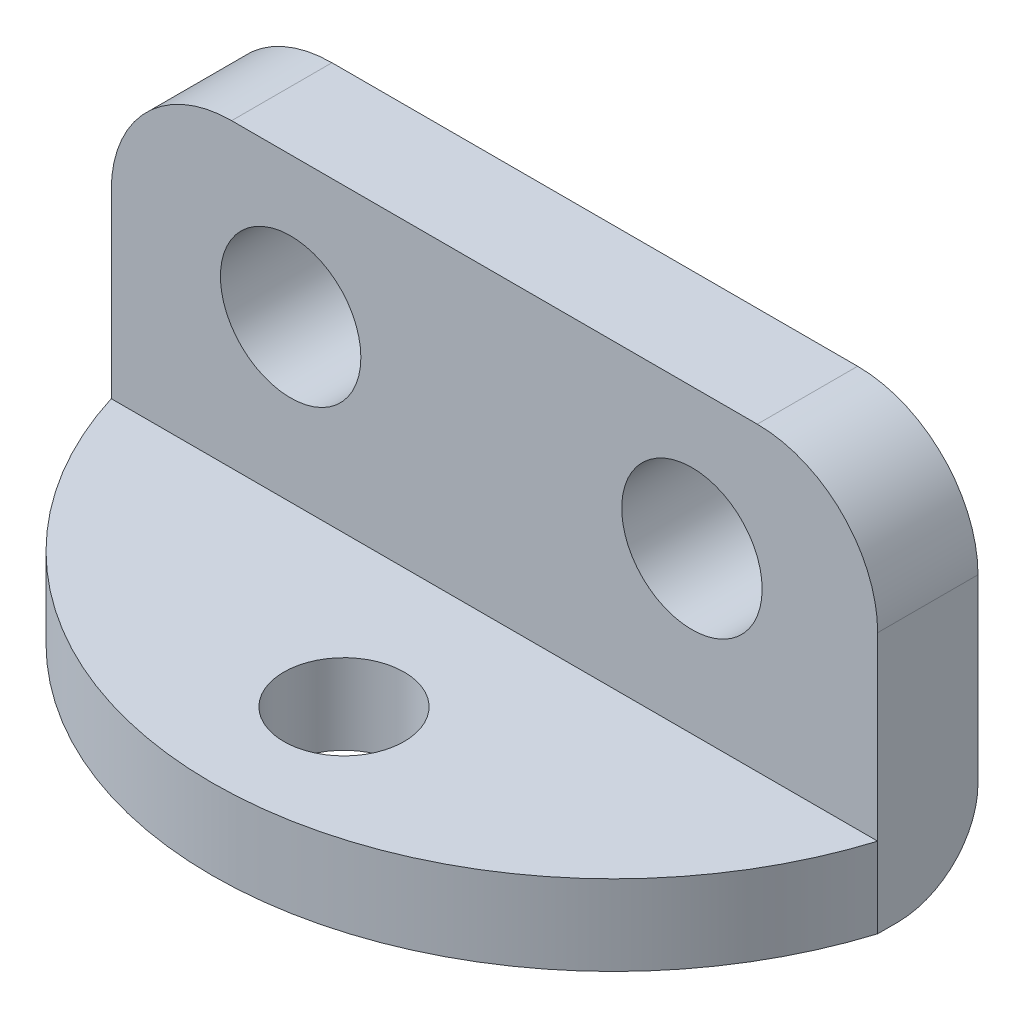
SolidWorks part; units mm, degrees
ref_plane "前视基准面" through (0, 0, 0) normal (0, 0, 1) x (1, 0, 0)
ref_plane "上视基准面" through (0, 0, 0) normal (0, 1, 0) x (1, 0, 0)
ref_plane "右视基准面" through (0, 0, 0) normal (1, 0, 0) x (0, 0, -1)
sketch "草图1" plane through (0, 0, 0) normal (0, 0, 1) x (1, 0, 0)
  line L0 (-0.0794, 0) -> (-0.0794, -3.7891) construction
  line L1 (-9.55, -4.75) -> (9.55, -4.75)
  line L2 (-9.55, -4.75) -> (-9.55, 1.75)
  line L3 (-6.55, 4.75) -> (6.55, 4.75)
  line L4 (9.55, -4.75) -> (9.55, 1.75)
  line L5 (-9.55, -4.75) -> (9.55, 4.75) construction
  line L6 (-9.55, 4.75) -> (9.55, -4.75) construction
  circle A0 centre (4.9206, 1.25) radius 1.75
  circle A1 centre (-5.0794, 1.25) radius 1.75
  arc A2 (6.55, 4.75) -> (9.55, 1.75) centre (6.55, 1.75) cw
  arc A3 (-9.55, 1.75) -> (-6.55, 4.75) centre (-6.55, 1.75) cw
  point P0 (0, 0)
  dimension "D5" = 3
  dimension "D6" = 3.5
  dimension "D1" = 19.1
  dimension "D2" = 9.5
  dimension "D3" = 3.5
  dimension "D4" = 10
extrude "凸台-拉伸1" add sketch "草图1" along normal blind 2.5
sketch "草图2" plane through (0, -4.75, 0) normal (0, -1, 0) x (1, 0, 0)
  line L0 (0, 1005.4255) -> (0, 2.5) construction
  line L1 (-9.55, 2.5) -> (9.55, 2.5)
  line L2 (6.55, 0) -> (-6.55, 0) construction
  arc A0 (9.55, 2.5) -> (-9.55, 2.5) centre (0, -0.4661) ccw
  circle A1 centre (0, 6.25) radius 1.5
  point P9 (9.55, 2.5)
  point P10 (-9.55, 2.5)
  dimension "D1" = 20
  dimension "D2" = 3
  dimension "D3" = 6.25
extrude "凸台-拉伸2" add sketch "草图2" against normal blind 2
fillet "圆角1" radius 2 1 edges at (0, -4.75, 0)
